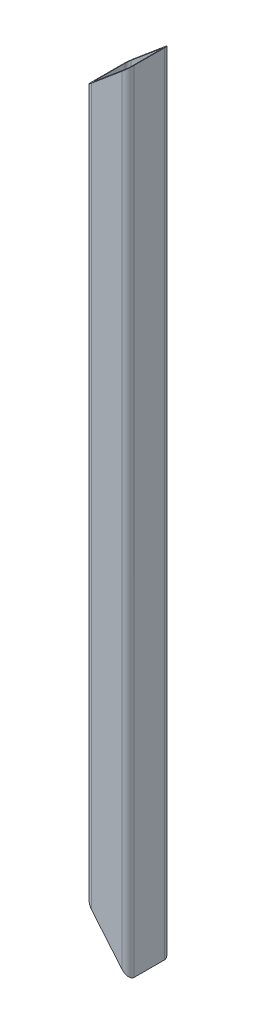
from build123d import *

# Parameters (mm, degrees)
FEATURE_19_WELDMEMBERFEAT_4_MORE_IN_5_DEPTH = 1302
CUT_EXTRUDE1_DEPTH                          = 1305.350029708
CUT_EXTRUDE1_DEPTH_BACK                     = 1305.350029708


with BuildPart() as part:
    # Sketch1 → feature 19 (WeldMemberFeat) (+4 more in 5 files) Cold-formed Hollow Structural Square Steel(gb t6728-2002) 70×70×5(1) (new body)
    with BuildSketch(Plane(origin=(0, 0, 0), x_dir=(-1, 0, 0), z_dir=(0, 1, 0))):
        with BuildLine():
            Line((-25, -35), (25, -35))
            ThreePointArc((25, -35), (32.071067812, -32.071067812), (35, -25))
            Line((35, -25), (35, 25))
            ThreePointArc((35, 25), (32.071067812, 32.071067812), (25, 35))
            Line((25, 35), (-25, 35))
            ThreePointArc((-25, 35), (-32.071067812, 32.071067812), (-35, 25))
            Line((-35, 25), (-35, -25))
            ThreePointArc((-35, -25), (-32.071067812, -32.071067812), (-25, -35))
        make_face()
        with BuildLine():
            Line((-25, -30), (25, -30))
            ThreePointArc((25, -30), (28.535533906, -28.535533906), (30, -25))
            Line((30, -25), (30, 25))
            ThreePointArc((30, 25), (28.535533906, 28.535533906), (25, 30))
            Line((25, 30), (-25, 30))
            ThreePointArc((-25, 30), (-28.535533906, 28.535533906), (-30, 25))
            Line((-30, 25), (-30, -25))
            ThreePointArc((-30, -25), (-28.535533906, -28.535533906), (-25, -30))
        make_face(mode=Mode.SUBTRACT)
    extrude(amount=FEATURE_19_WELDMEMBERFEAT_4_MORE_IN_5_DEPTH)

    # 0:feat:20/0 feature 20/0 (ProfileFeature) (+11 more in 7 files) Sketch2 → Cut-Extrude1 (cut, two sides: drawn at the far end of the back side and taken through both)
    with BuildSketch(Plane.XY.offset(35).offset(-CUT_EXTRUDE1_DEPTH_BACK)):
        Polygon((35, 1302), (-35, 1243.247002398), (-35, 1302), align=None)
        Polygon((-35, 83.4), (35, 0), (-35, 0), align=None)
    extrude(amount=CUT_EXTRUDE1_DEPTH + CUT_EXTRUDE1_DEPTH_BACK, mode=Mode.SUBTRACT)


solid = part.part
